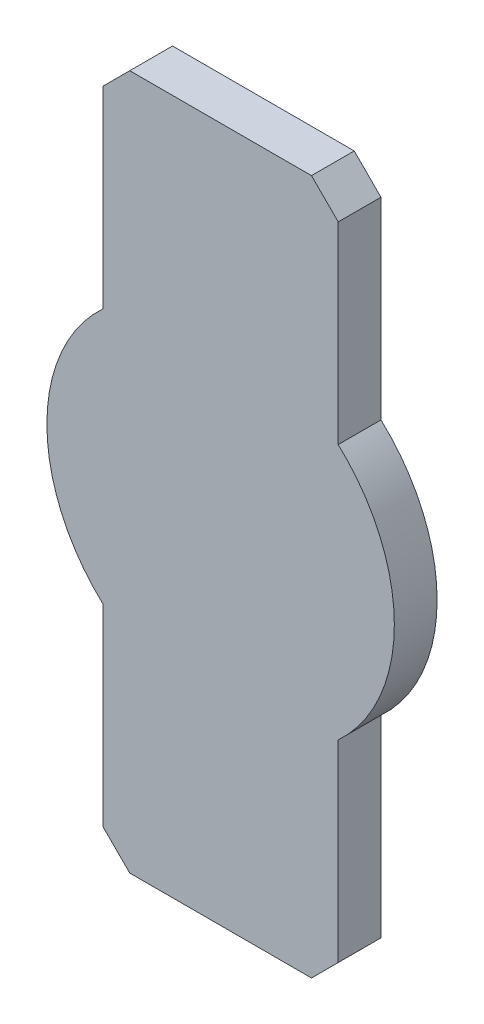
from build123d import *

# Parameters (mm, degrees)
SKETCH_1_R      = 32.5
EXTRUDE_1_DEPTH = 4
SKETCH_2_W      = 44
SKETCH_2_H      = 130
EXTRUDE_2_DEPTH = 8
CHAMFER_1_SIZE  = 5


with BuildPart() as part:
    # 草图1 → 凸台-拉伸1 (new, symmetric)
    with BuildSketch(Plane.XY):
        Circle(SKETCH_1_R)
    extrude(amount=EXTRUDE_1_DEPTH, both=True)

    # 草图2 → 凸台-拉伸2 (add)
    with BuildSketch(Plane.XY.offset(4)):
        Rectangle(SKETCH_2_W, SKETCH_2_H)
    extrude(amount=-EXTRUDE_2_DEPTH)

    # 倒角1
    chamfer_1_edges = [part.edges().sort_by_distance(p)[0] for p in [
        (22, 65, 0),
        (-22, -65, 0),
        (22, -65, 0),
        (-22, 65, 0),
    ]]
    chamfer(chamfer_1_edges, length=CHAMFER_1_SIZE)


solid = part.part
